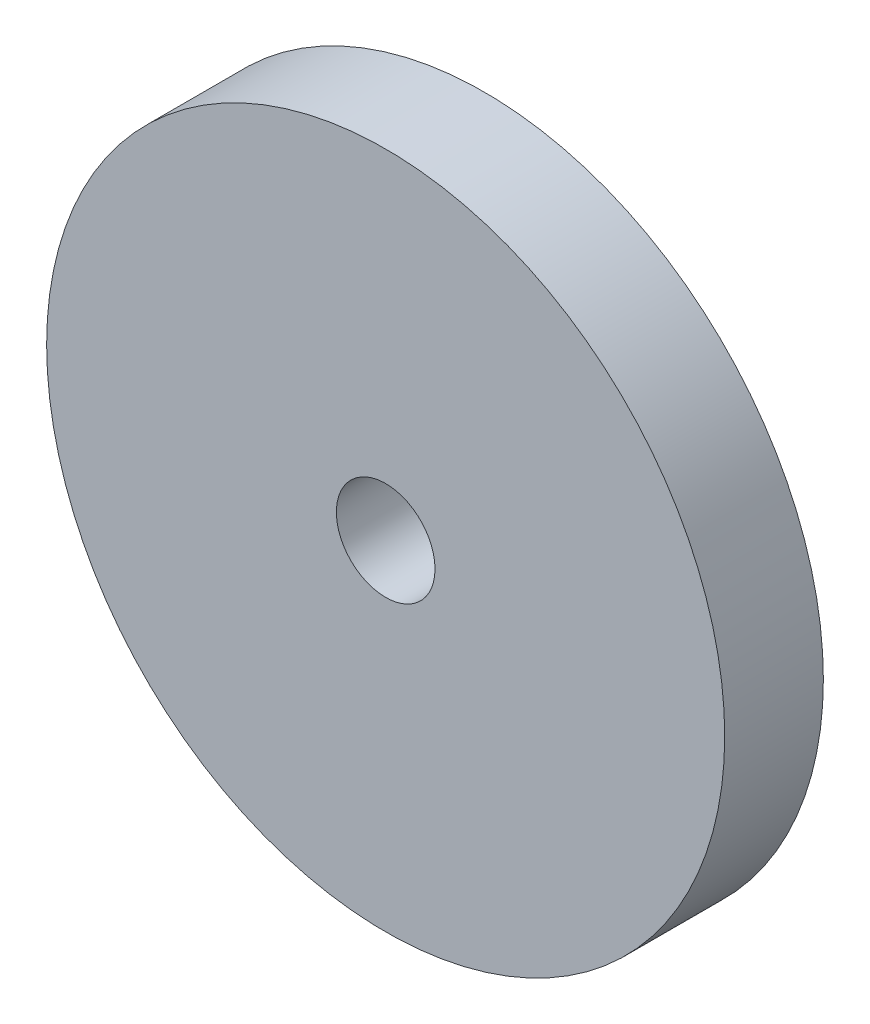
SolidWorks part; units mm, degrees
material "1023 Carbon steel plate (SS)"
ref_plane "Front Plane" through (0, 0, 0) normal (0, 0, 1) x (1, 0, 0)
ref_plane "Top Plane" through (0, 0, 0) normal (0, 1, 0) x (1, 0, 0)
ref_plane "Right Plane" through (0, 0, 0) normal (1, 0, 0) x (0, 0, -1)
sketch "Sketch1" plane through (0, 0, 0) normal (0, 0, 1) x (1, 0, 0)
  circle A0 centre (0, 0) radius 41.25
  circle A2 centre (0, 0) radius 6
  dimension "D1" = 82.5
  dimension "D2" = 12
extrude "Boss-Extrude1" add sketch "Sketch1" along normal blind 12 contours A0 | A2
